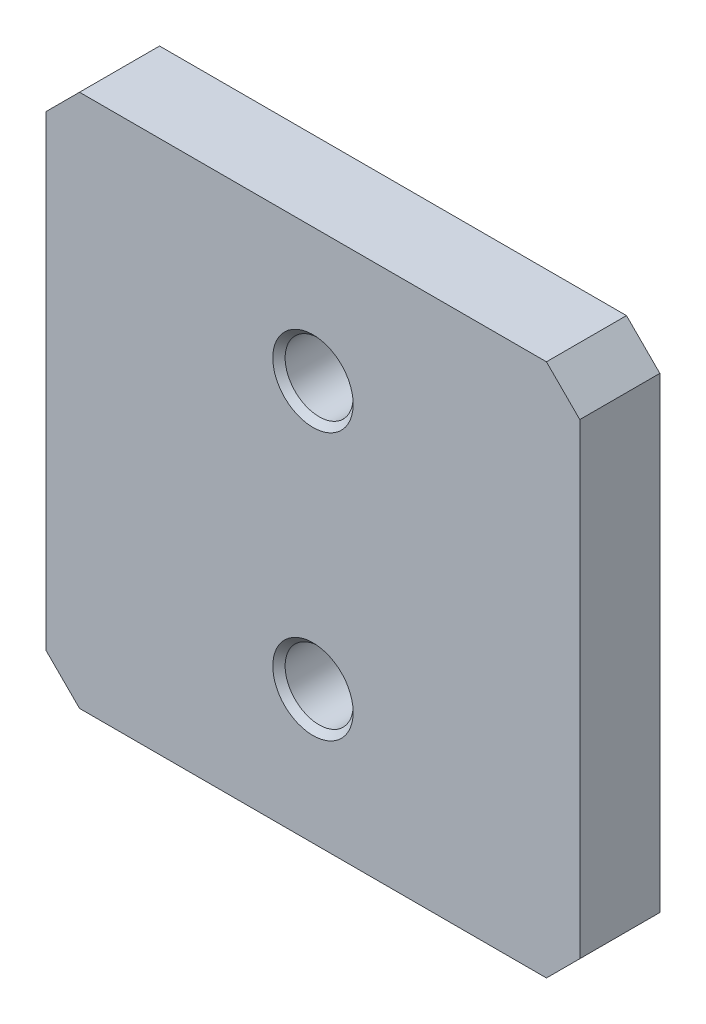
SolidWorks part; units mm, degrees
material "Q235-A "
ref_plane "前视基准面" through (0, 0, 0) normal (0, 0, 1) x (1, 0, 0)
ref_plane "上视基准面" through (0, 0, 0) normal (0, 1, 0) x (1, 0, 0)
ref_plane "右视基准面" through (0, 0, 0) normal (1, 0, 0) x (0, 0, -1)
sketch "草图1" plane through (0, 0, 0) normal (0, 0, 1) x (1, 0, 0)
  line L1 (-40, 40) -> (40, 40)
  line L2 (-40, 40) -> (-40, -40)
  line L3 (-40, -40) -> (40, -40)
  line L4 (40, 40) -> (40, -40)
  line L5 (-40, 40) -> (40, -40) construction
  line L6 (-40, -40) -> (40, 40) construction
  point P0 (0, 0)
  dimension "D1" = 80
  dimension "D2" = 80
extrude "凸台-拉伸1" add sketch "草图1" along normal blind 12
chamfer "倒角1" distance 5 angle 45 4 edges at (40, -40, 6) (-40, -40, 6) (40, 40, 6) (-40, 40, 6)
sketch "草图2" plane through (0, 0, 12) normal (0, 0, 1) x (1, 0, 0)
  line L0 (0, 40) -> (0, -40) construction
  line L1 (35, 40) -> (-35, 40) construction
  line L2 (-35, -40) -> (35, -40) construction
  line L3 (0, 0) -> (40, 0) construction
  line L4 (40, -35) -> (40, 35) construction
  circle A0 centre (0, 20) radius 2.5
  circle A1 centre (0, -20) radius 2.5
  dimension "D1" = 5
  dimension "D2" = 40
hole_wizard "M12 螺纹孔1" positions "3D草图1" profile "草图3" tap size "M12" standard "GB"
sketch3d "3D草图1"
  point P0 (0, 20, 12)
  point P3 (0, -20, 12)
sketch "草图3" plane through (0, 20, 12) normal (1, 0, 0) x (0, -1, 0)
  line L0 (0, 0) -> (0, 35.8144)
  line L1 (0, 35.8144) -> (5.1, 32.75)
  line L2 (5.1, 32.75) -> (5.1, 0.925)
  line L3 (5.1, 0.925) -> (6.025, 0)
  line L5 (6.025, 0) -> (0, 0)
  line L6 (-5.1, 0.925) -> (-6.025, 0) construction
  line L10 (0, 35.8144) -> (-5.1, 32.75) construction
  line L11 (0, -6.35) -> (0, 107.95) construction
  dimension "螺纹孔钻头直径" = 10.2
  dimension "螺纹孔钻头深度" = 32.75
  dimension "近端锥形沉头孔直径" = 12.05
  dimension "近端锥形沉头孔角度" = 90
  dimension "导头角度" = 118
cosmetic thread "孔螺蚊线1" parameters "D1"=10, "D2"=12
cosmetic thread "孔螺蚊线2" parameters "D1"=10, "D2"=12
